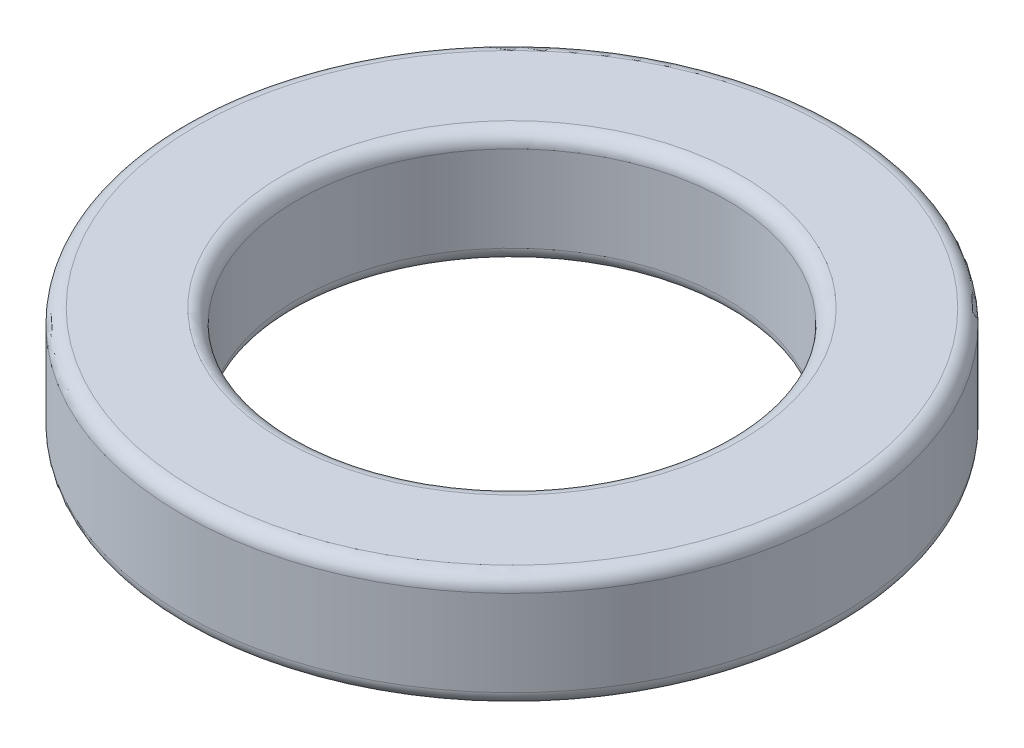
SolidWorks part; units mm, degrees
material "AISI 304"
ref_plane "前视基准面" through (0, 0, 0) normal (0, 0, 1) x (1, 0, 0)
ref_plane "上视基准面" through (0, 0, 0) normal (0, 1, 0) x (1, 0, 0)
ref_plane "右视基准面" through (0, 0, 0) normal (1, 0, 0) x (0, 0, -1)
sketch "草图1" plane through (0, 0, 0) normal (0, 1, 0) x (1, 0, 0)
  circle A0 centre (0, 0) radius 2.3
  circle A1 centre (0, 0) radius 1.5
  dimension "D1" = 3
  dimension "D2" = 4.6
extrude "凸台-拉伸1" add sketch "草图1" along normal blind 0.8
fillet "圆角1" radius 0.1 4 edges at (0, 0, 1.5) (0, 0, 2.3) (0, 0.8, 1.5) (0, 0.8, 2.3)
